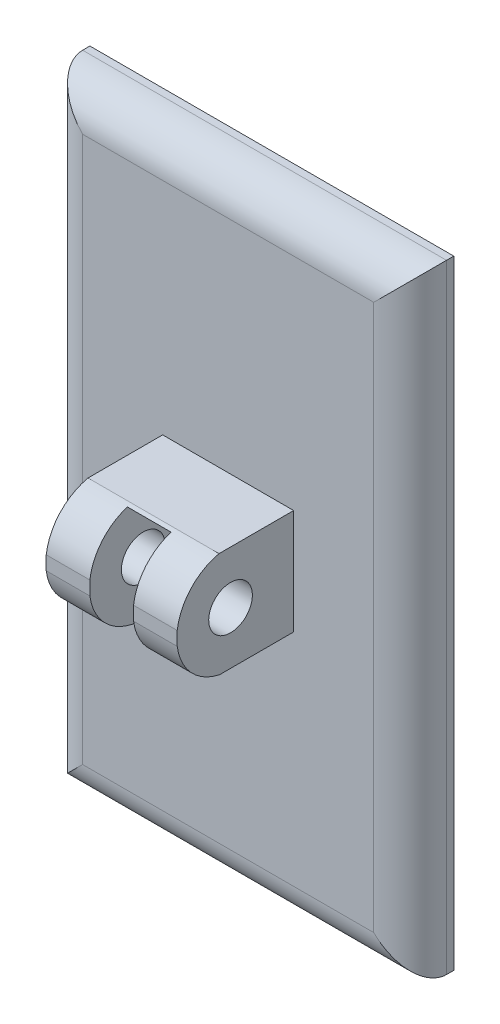
SolidWorks part; units mm, degrees
ref_plane "Front Plane" through (0, 0, 0) normal (0, 0, 1) x (1, 0, 0)
ref_plane "Top Plane" through (0, 0, 0) normal (0, 1, 0) x (1, 0, 0)
ref_plane "Right Plane" through (0, 0, 0) normal (1, 0, 0) x (0, 0, -1)
other "Configuration Table"
sketch "Sketch1" plane through (0, 0, 0) normal (0, 0, 1) x (1, 0, 0)
  line L1 (0, 0) -> (50, 0)
  line L2 (0, 0) -> (0, 85)
  line L3 (0, 85) -> (50, 85)
  line L4 (50, 0) -> (50, 85)
  dimension "D1" = 85
  dimension "D2" = 50
extrude "Boss-Extrude1" add sketch "Sketch1" along normal blind 6
sketch "Sketch2" plane through (0, 0, 6) normal (0, 0, 1) x (1, 0, 0)
  line L0 (0, 85) -> (0, 0) construction
  line L1 (16, 49.7242) -> (34, 49.7242)
  line L2 (16, 49.7242) -> (16, 35.2758)
  line L3 (16, 35.2758) -> (34, 35.2758)
  line L4 (34, 49.7242) -> (34, 35.2758)
  line L5 (16, 49.7242) -> (34, 35.2758) construction
  line L6 (16, 35.2758) -> (34, 49.7242) construction
  line L7 (25, 85) -> (25, 0) construction
  line L8 (50, 85) -> (0, 85) construction
  line L9 (0, 0) -> (50, 0) construction
  line L10 (0, 42.5) -> (50, 42.5) construction
  line L11 (50, 0) -> (50, 85) construction
  point P0 (25, 42.5)
  dimension "D1" = 18
extrude "Boss-Extrude2" add sketch "Sketch2" along normal blind 16
fillet "Fillet1" radius 5 4 edges at (25, 0, 6) (50, 42.5, 6) (25, 85, 6) (0, 42.5, 6)
sketch "Sketch3" plane through (0, 0, 22) normal (0, 0, 1) x (1, 0, 0)
  line L0 (16, 49.7242) -> (16, 35.2758) construction
  line L1 (22, 49.5702) -> (28, 49.5702)
  line L2 (22, 49.5702) -> (22, 19.8537)
  line L3 (22, 19.8537) -> (28, 19.8537)
  line L4 (28, 49.5702) -> (28, 19.8537)
  line L5 (22, 49.5702) -> (28, 19.8537) construction
  line L6 (22, 19.8537) -> (28, 49.5702) construction
  point P0 (25, 34.712)
  dimension "D1" = 6
  dimension "D2" = 9
extrude "Cut-Extrude1" cut sketch "Sketch3" against normal blind 16
sketch "Sketch4" plane through (16, 0, 0) normal (-1, 0, 0) x (0, 0, 1)
  line L0 (14.6733, 49.8958) -> (20.8021, 55.1158)
  line L1 (20.8021, 55.1158) -> (35.7981, 48.4028)
  line L2 (35.7981, 48.4028) -> (20.2128, 12.7107)
  line L3 (20.2128, 12.7107) -> (14.6733, 35.1199)
  circle A0 centre (14.6733, 42.5078) radius 3
  arc A1 (14.6733, 35.1199) -> (14.6733, 49.8958) centre (14.6733, 42.5078) ccw
  dimension "D1" = 6
extrude "Cut-Extrude2" cut sketch "Sketch4" against normal through all
